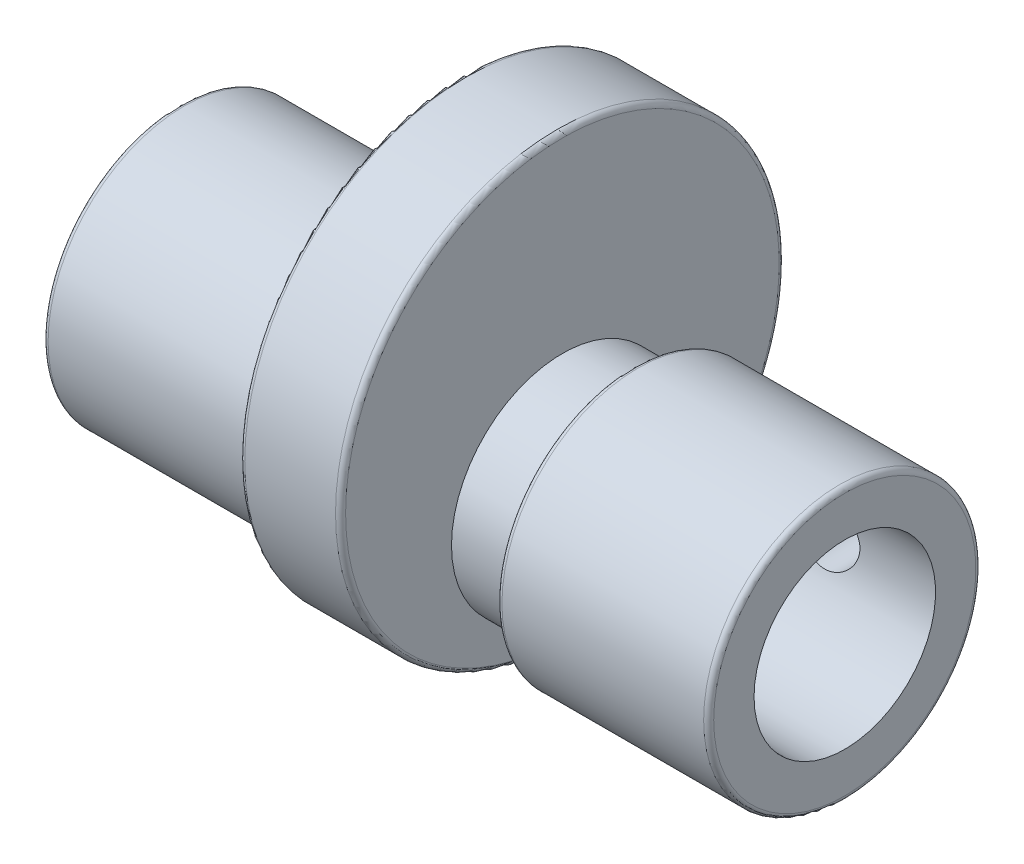
SolidWorks part; units mm, degrees
ref_plane "Front Plane" through (0, 0, 0) normal (0, 0, 1) x (1, 0, 0)
ref_plane "Top Plane" through (0, 0, 0) normal (0, 1, 0) x (1, 0, 0)
ref_plane "Right Plane" through (0, 0, 0) normal (1, 0, 0) x (0, 0, -1)
sketch "Sketch1" plane through (0, 0, 0) normal (0, 0, 1) x (1, 0, 0)
  line L0 (0, 0) -> (66, 0) construction
  line L1 (0, 9) -> (0, 13.5)
  line L2 (0, 13.5) -> (21, 13.5)
  line L3 (21, 13.5) -> (21, 11)
  line L4 (21, 11) -> (45, 11)
  line L5 (45, 11) -> (45, 13.5)
  line L6 (45, 13.5) -> (66, 13.5)
  line L7 (66, 13.5) -> (66, 9)
  line L8 (0, 9) -> (15, 9)
  line L9 (15, 9) -> (15, 8)
  line L10 (15, 8) -> (51, 8)
  line L11 (51, 8) -> (51, 9)
  line L12 (51, 9) -> (66, 9)
  point P17 (33, 8)
  point P18 (33, 11)
  dimension "D1" = 66
  dimension "D2" = 24
  dimension "D3" = 13.5
  dimension "D4" = 11
  dimension "D5" = 9
  dimension "D6" = 8
  dimension "D7" = 36
revolve "Revolve1" add sketch "Sketch1" angle 360 about L0
ref_plane "Plane1" through (33, 0, 0) normal (-1, 0, 0) x (0, 0, 1)
sketch "Sketch2" plane through (33, 0, 0) normal (-1, 0, 0) x (0, 0, 1)
  line L0 (0, 30) -> (7.1674, 30) construction
  circle A0 centre (0, 8) radius 22
  dimension "D1" = 44
  dimension "D2" = 30
extrude "Boss-Extrude1" add sketch "Sketch2" against normal mid plane 10
sketch "Sketch3" plane through (38, 0, 0) normal (1, 0, 0) x (0, 0, -1)
  circle A1 centre (0, 0) radius 8
  circle A2 centre (0, 0) radius 8
  dimension "D1" = 0
extrude "Cut-Extrude1" cut sketch "Sketch3" against normal mid plane 26
fillet "Fillet1" radius 0.5 6 edges at (66, 0, 13.5) (45, 0, 13.5) (28, 8, 22) (38, 8, 22) (21, 0, 13.5) (0, 0, 13.5)
sketch "Sketch4" plane through (0, 0, 0) normal (0, 0, 1) x (1, 0, 0)
  line L0 (66, -13) -> (66, 13) construction
  circle A0 centre (55.5, 0) radius 3
  dimension "D2" = 6
  dimension "D1" = 10.5
extrude "Cut-Extrude2" cut sketch "Sketch4" against normal blind 26
